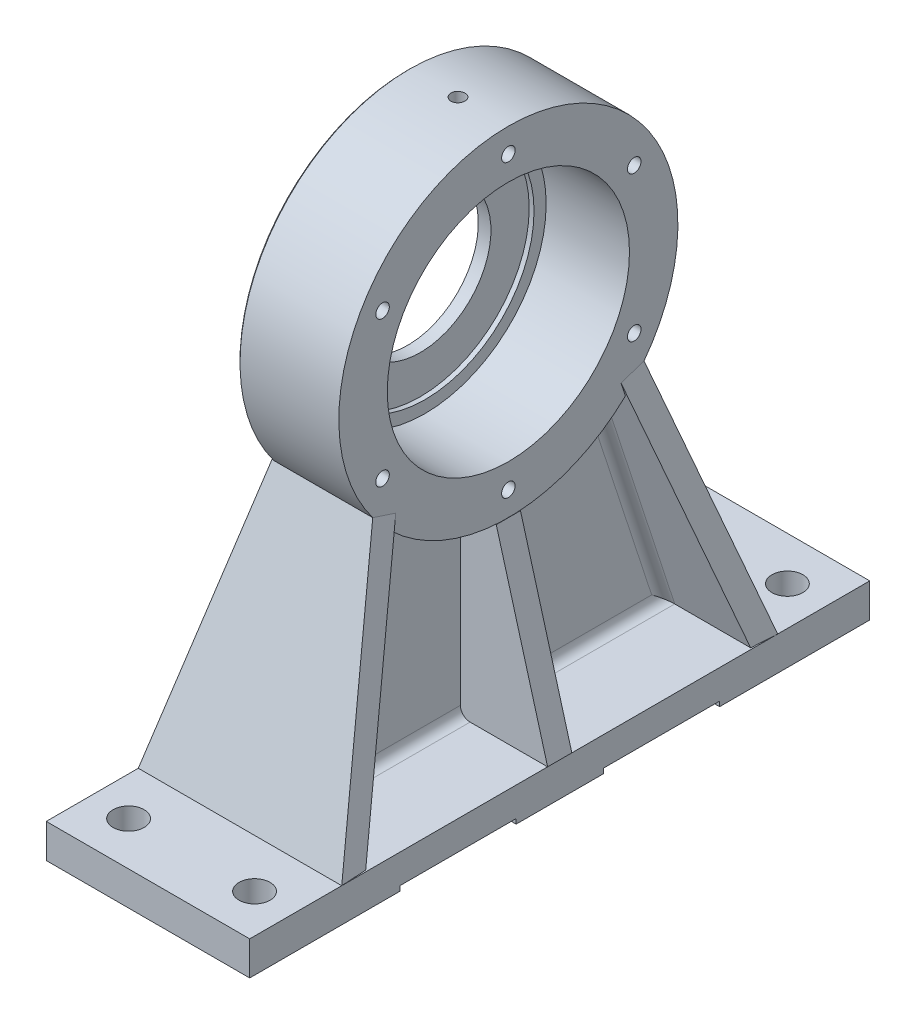
SolidWorks part; units mm, degrees
material "HT200"
ref_plane "Front Plane" through (0, 0, 0) normal (0, 0, 1) x (1, 0, 0)
ref_plane "Top Plane" through (0, 0, 0) normal (0, 1, 0) x (1, 0, 0)
ref_plane "Right Plane" through (0, 0, 0) normal (1, 0, 0) x (0, 0, -1)
sketch "Sketch1" plane through (0, 0, 0) normal (0, 0, 1) x (1, 0, 0)
  line L0 (0, 0) -> (123.5206, 0) construction
  line L1 (-52, 73) -> (-52, 175)
  line L2 (-52, 175) -> (52, 175)
  line L3 (52, 175) -> (52, 125)
  line L4 (52, 125) -> (-34, 125)
  line L5 (-34, 125) -> (-34, 112.5)
  line L6 (-39, 73) -> (-52, 73)
  line L7 (-34, 112.5) -> (-39, 112.5)
  line L8 (-39, 112.5) -> (-39, 73)
  point P9 (0, 175)
  dimension "D1" = 104
  dimension "D2" = 86
  dimension "D3" = 146
  dimension "D4" = 250
  dimension "D5" = 350
  dimension "D6" = 225
  dimension "D7" = 5
revolve "Revolve1" add sketch "Sketch1" angle 360 about L0
sketch "Sketch2" plane through (0, 0, 0) normal (1, 0, 0) x (0, 0, -1)
  line L0 (-320, -400) -> (-320, -365)
  line L1 (-320, -365) -> (320, -365)
  line L2 (320, -365) -> (320, -400)
  line L3 (320, -400) -> (165, -400)
  line L4 (165, -400) -> (165, -395)
  line L5 (165, -395) -> (45, -395)
  line L6 (45, -395) -> (45, -400)
  line L7 (45, -400) -> (-45, -400)
  line L8 (-45, -400) -> (-45, -395)
  line L9 (-45, -395) -> (-165, -395)
  line L10 (-165, -395) -> (-165, -400)
  line L11 (-165, -400) -> (-320, -400)
  line L12 (0, 0) -> (0, -400) construction
  point P15 (0, -365)
  dimension "D1" = 400
  dimension "D2" = 640
  dimension "D3" = 120
  dimension "D4" = 5
  dimension "D5" = 90
  dimension "D6" = 35
extrude "Boss-Extrude1" add sketch "Sketch2" along normal mid plane 210 separate body
sketch "Sketch3" plane through (0, 0, 0) normal (1, 0, 0) x (0, 0, -1)
  line L0 (-140, -105) -> (-225, -365)
  line L1 (320, -365) -> (-320, -365) construction
  line L2 (-225, -365) -> (225, -365)
  line L3 (225, -365) -> (140, -105)
  line L4 (0, 0) -> (0, -455.4927) construction
  line L5 (-320, -365) -> (-320, -400) construction
  circle A0 centre (0, 0) radius 175 construction
  arc A1 (140, -105) -> (-140, -105) centre (0, 0) cw
  dimension "D1" = 95
  dimension "D2" = 280
extrude "Boss-Extrude2" add sketch "Sketch3" along normal mid plane 30
sketch "Sketch6" plane through (0, 0, 0) normal (0, 0, 1) x (1, 0, 0)
  line L0 (-52, -175) -> (-105, -365)
  line L1 (-52, 175) -> (-52, -175) construction
  line L2 (-105, -365) -> (105, -365)
  line L3 (105, -365) -> (52, -175)
  line L4 (52, -175) -> (52, 175) construction
  line L5 (52, -175) -> (-52, -175)
  line L6 (15, -175) -> (52, -175) construction
extrude "Boss-Extrude6" add sketch "Sketch6" along normal mid plane 25 separate body contours L3 L5 L0 L2
sketch "Sketch4" plane through (0, 31.2112, 95.4694) normal (0, 0.3107, 0.9505) x (1, 0, 0)
  line L0 (-52, -143.3054) -> (52, -143.3054)
  line L1 (52, -143.3054) -> (105, -416.847)
  line L2 (105, -416.847) -> (-105, -416.847)
  line L3 (-105, -416.847) -> (-52, -143.3054)
  line L4 (15, -143.3054) -> (-15, -143.3054) construction
  line L5 (15, -416.847) -> (-15, -416.847) construction
  line L6 (-105, -247.4944) -> (-105, -446.3672) construction
  line L7 (-52, 175) -> (-52, -175) construction
  point P6 (0, -143.3054)
  point P8 (0, -416.847)
extrude "Boss-Extrude3" add sketch "Sketch4" against normal blind 25
mirror "Mirror1" about plane through (0, 0, 0) normal (0, 0, 1) of "Boss-Extrude3"
fillet "Fillet1" radius 10 7 edges at (-15, -365, 0) (-15, -245.822, -159.7359) (-15, -175, 0) (15, -245.822, -159.7359) (15, -365, 0) (15, -245.822, 159.7359) (15, -175, 0)
sketch "Sketch7" plane through (0, -365, 0) normal (0, 1, 0) x (1, 0, 0)
  line L1 (-65, 275) -> (65, 275) construction
  line L2 (-65, 275) -> (-65, -275) construction
  line L3 (-65, -275) -> (65, -275) construction
  line L4 (65, 275) -> (65, -275) construction
  line L5 (-65, 275) -> (65, -275) construction
  line L6 (-65, -275) -> (65, 275) construction
  circle A0 centre (-65, 275) radius 16
  circle A1 centre (65, 275) radius 16
  circle A2 centre (-65, -275) radius 16
  circle A3 centre (65, -275) radius 16
  point P0 (0, 0)
  dimension "D1" = 32
  dimension "D2" = 130
  dimension "D3" = 550
extrude "Cut-Extrude1" cut sketch "Sketch7" against normal through all
sketch "Sketch8" plane through (52, 0, 0) normal (1, 0, 0) x (0, 0, -1)
  circle A0 centre (0, 0) radius 150
  circle A1 centre (0, 150) radius 6
  circle A2 centre (129.9038, 75) radius 6
  circle A3 centre (129.9038, -75) radius 6
  circle A4 centre (0, -150) radius 6
  circle A5 centre (-129.9038, -75) radius 6
  circle A6 centre (-129.9038, 75) radius 6
  dimension "D1" = 300
  dimension "D2" = 12
  dimension "D3" = 6
hole_wizard "M16 Tapped Hole1" positions "Sketch10" profile "Sketch9" tap size "M16" standard "GB"
sketch "Sketch10" plane through (52, 0, 0) normal (1, 0, 0) x (0, 0, -1)
  point P0 (-129.9038, -75)
  point P1 (0, -150)
  point P4 (129.9038, -75)
  point P7 (129.9038, 75)
  point P10 (0, 150)
  point P13 (-129.9038, 75)
sketch "Sketch9" plane through (52, -75, 129.9038) normal (0, 1, 0) x (0, 0, -1)
  line L0 (0, 0) -> (0, 42.206)
  line L1 (0, 42.206) -> (7, 38)
  line L2 (7, 38) -> (7, 0)
  line L5 (7, 0) -> (0, 0)
  line L10 (0, 42.206) -> (-7, 38) construction
  line L11 (0, -6.35) -> (0, 107.95) construction
  dimension "螺纹孔钻头直径" = 14
  dimension "螺纹孔钻头深度" = 38
  dimension "导头角度" = 118
cosmetic thread "Cosmetic Thread 1" parameters "D1"=32, "D2"=16
cosmetic thread "Cosmetic Thread 2" parameters "D1"=32, "D2"=16
cosmetic thread "Cosmetic Thread 3" parameters "D1"=32, "D2"=16
cosmetic thread "Cosmetic Thread 4" parameters "D1"=32, "D2"=16
cosmetic thread "Cosmetic Thread 5" parameters "D1"=32, "D2"=16
cosmetic thread "Cosmetic Thread 6" parameters "D1"=32, "D2"=16
ref_plane "Plane1" through (0, 175, 0) normal (0, 1, 0) x (-1, 0, 0)
sketch "Sketch11" plane through (0, 175, 0) normal (0, 1, 0) x (-1, 0, 0)
  point P0 (0, 0)
hole_wizard "M16x1.5 Tapped Hole1" positions "3DSketch1" profile "Sketch12" tap size "M16x1.5" standard "GB"
sketch3d "3DSketch1"
  point P0 (0, 175, 0)
sketch "Sketch12" plane through (0, 175, 0) normal (1, 0, 0) x (0, 0, 1)
  line L0 (0, 0) -> (0, 60.8562)
  line L1 (0, 60.8562) -> (7.25, 56.5)
  line L2 (7.25, 56.5) -> (7.25, 0)
  line L5 (7.25, 0) -> (0, 0)
  line L10 (0, 60.8562) -> (-7.25, 56.5) construction
  line L11 (0, -6.35) -> (0, 107.95) construction
  dimension "螺纹孔钻头直径" = 14.5
  dimension "螺纹孔钻头深度" = 56.5
  dimension "导头角度" = 118
cosmetic thread "Cosmetic Thread 7" parameters "D1"=32, "D2"=16
chamfer "Chamfer1" distance 2 angle 45 1 edges at (-52, 175, 0)
